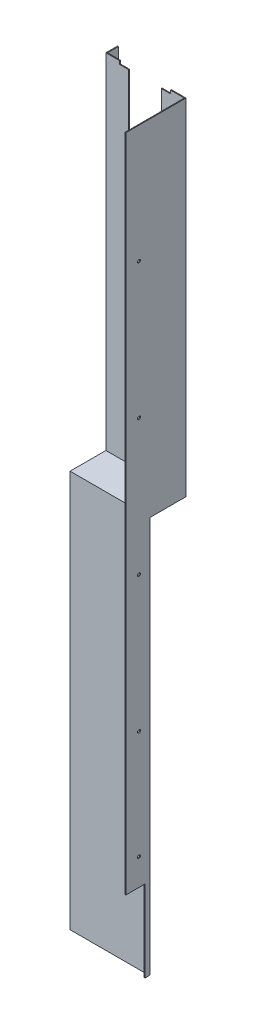
SolidWorks part; units mm, degrees
ref_plane "前视基准面" through (0, 0, 0) normal (0, 0, 1) x (1, 0, 0)
ref_plane "上视基准面" through (0, 0, 0) normal (0, 1, 0) x (1, 0, 0)
ref_plane "右视基准面" through (0, 0, 0) normal (1, 0, 0) x (0, 0, -1)
sketch "草图1" plane through (0, 0, 0) normal (0, 0, 1) x (1, 0, 0)
  line L1 (0, 0) -> (146, 0)
  line L2 (0, 0) -> (0, 636)
  line L3 (0, 636) -> (146, 636)
  line L4 (146, 0) -> (146, 636)
  dimension "D1" = 146
  dimension "D2" = 636
extrude "凸台-拉伸1" add sketch "草图1" along normal blind 1.5
sketch "草图3" plane through (0, 0, 1.5) normal (0, 0, 1) x (1, 0, 0)
  line L0 (0, 0) -> (146, 0) construction
  line L1 (146, 636) -> (144.5, 636)
  line L2 (146, 636) -> (146, 0)
  line L3 (146, 0) -> (144.5, 0)
  line L4 (144.5, 636) -> (144.5, 0)
  dimension "D1" = 1.5
extrude "凸台-拉伸3" add sketch "草图3" along normal blind 109
sketch "草图4" plane through (0, 0, 1.5) normal (0, 0, 1) x (1, 0, 0)
  line L0 (144.5, 636) -> (144.5, 0) construction
  line L1 (0, 0) -> (144.5, 0)
  line L2 (0, 0) -> (0, 1.5)
  line L3 (0, 1.5) -> (144.5, 1.5)
  line L4 (144.5, 0) -> (144.5, 1.5)
  dimension "D1" = 1.5
extrude "凸台-拉伸4" add sketch "草图4" along normal blind 66
sketch "草图5" plane through (0, 0, 0) normal (0, -1, 0) x (1, 0, 0)
  line L0 (0, 67.5) -> (144.5, 67.5)
  line L1 (0, 67.5) -> (144.5, 67.5) construction
  line L2 (144.5, 110.5) -> (144.5, 67.5) construction
  line L3 (144.5, 67.5) -> (144.5, 110.5)
  line L4 (144.5, 110.5) -> (146, 110.5)
  line L5 (146, 110.5) -> (146, 66)
  line L6 (146, 110.5) -> (146, 0) construction
  line L7 (146, 66) -> (0, 66)
  line L8 (0, 67.5) -> (0, 0) construction
  line L9 (0, 66) -> (0, 67.5)
  dimension "D1" = 1.5
extrude "凸台-拉伸5" add sketch "草图5" along normal blind 730
sketch "草图6" plane through (0, 0, 0) normal (0, 0, -1) x (-1, 0, 0)
  line L1 (0, 636) -> (-1.5, 636)
  line L2 (0, 636) -> (0, 1.5)
  line L3 (0, 1.5) -> (-1.5, 1.5)
  line L4 (-1.5, 636) -> (-1.5, 1.5)
  line L5 (0, 0) -> (-146, 0) construction
  dimension "D1" = 1.5
  dimension "D2" = 1.5
extrude "凸台-拉伸6" add sketch "草图6" along normal blind 20
sketch "草图7" plane through (0, 0, 66) normal (0, 0, -1) x (-1, 0, 0)
  line L0 (0, -730) -> (-146, -730) construction
  line L1 (0, 0) -> (-1.5, 0)
  line L2 (0, 0) -> (0, -730)
  line L3 (0, -730) -> (-1.5, -730)
  line L4 (-1.5, 0) -> (-1.5, -730)
  dimension "D1" = 1.5
extrude "凸台-拉伸7" add sketch "草图7" along normal blind 10
sketch "草图8" plane through (0, 0, 0) normal (0, -1, 0) x (1, 0, 0)
  line L1 (1.5, 56) -> (0, 56)
  line L2 (1.5, 56) -> (1.5, 0)
  line L3 (1.5, 0) -> (0, 0)
  line L4 (0, 56) -> (0, 0)
extrude "凸台-拉伸8" add sketch "草图8" along normal blind 10
sketch "草图9" plane through (144.5, 0, 0) normal (-1, 0, 0) x (0, 0, 1)
  line L1 (110.5, -730) -> (75.5, -730)
  line L2 (110.5, -730) -> (110.5, -580)
  line L3 (110.5, -580) -> (75.5, -580)
  line L4 (75.5, -730) -> (75.5, -580)
  dimension "D1" = 150
  dimension "D2" = 35
extrude "切除-拉伸1" cut sketch "草图9" against normal blind 2
sketch "草图10" plane through (0, 0, 1.5) normal (0, 0, 1) x (1, 0, 0)
  line L0 (0, 636) -> (0, 1.5) construction
  line L1 (25, 636) -> (119, 636)
  line L2 (119, 636) -> (119, 630)
  line L3 (25, 630) -> (42, 630)
  line L4 (25, 636) -> (25, 630)
  line L6 (42, 630) -> (42, 501)
  line L7 (42, 501) -> (102, 501)
  line L8 (102, 630) -> (102, 501)
  line L9 (102, 630) -> (119, 630)
  dimension "D1" = 94
  dimension "D2" = 6
  dimension "D3" = 60
  dimension "D4" = 17
  dimension "D5" = 135
  dimension "D6" = 17
  dimension "D7" = 25
extrude "切除-拉伸2" cut sketch "草图10" against normal blind 2
hole_wizard "Ø5.5 (5.5) 直径孔1" positions "草图12" profile "草图11" hole size "Ø5.5" standard "GB" end condition through all
sketch "草图12" plane through (144.5, 0, 0) normal (-1, 0, 0) x (0, 0, 1)
  line L1 (86.5, 636) -> (86.5, -907.068) construction
  line L2 (110.5, 636) -> (1.5, 636) construction
  line L4 (110.5, 636) -> (110.5, -580) construction
  point P0 (86.5, 419)
  point P1 (86.5, 169)
  point P3 (86.5, -81)
  point P5 (86.5, -331)
  point P13 (86.5, -531)
  dimension "D1" = 24
  dimension "D2" = 217
  dimension "D3" = 250
  dimension "D4" = 250
  dimension "D5" = 250
  dimension "D6" = 200
sketch "草图11" plane through (144.5, 419, 86.5) normal (0, 1, 0) x (0, 0, 1)
  line L0 (0, 0) -> (0, 1.5001)
  line L1 (0, 1.5001) -> (2.75, 1.5001)
  line L2 (2.75, 1.5001) -> (2.75, 0)
  line L5 (2.75, 0) -> (0, 0)
  line L11 (0, -6.35) -> (0, 107.95) construction
  dimension "通孔孔直径" = 5.5
  dimension "通孔孔深度" = 1.5001
hole_wizard "Ø5.5 (5.5) 直径孔2" positions "草图14" profile "草图13" hole size "Ø5.5" standard "GB" end condition through all
sketch "草图14" plane through (0, 0, 0) normal (-1, 0, 0) x (0, 0, 1)
  line L0 (-10, 636) -> (-10, -161.2553) construction
  line L1 (1.5, 636) -> (-20, 636) construction
  line L3 (-20, 1.5) -> (-20, 636) construction
  line L4 (-20, 1.5) -> (0, 1.5) construction
  point P0 (-10, 301.5)
  point P1 (-10, 101.5)
  dimension "D1" = 10
  dimension "D2" = 200
  dimension "D3" = 100
sketch "草图13" plane through (0, 301.5, -10) normal (0, 1, 0) x (0, 0, 1)
  line L0 (0, 0) -> (0, 146.0001)
  line L1 (0, 146.0001) -> (2.75, 146.0001)
  line L2 (2.75, 146.0001) -> (2.75, 0)
  line L5 (2.75, 0) -> (0, 0)
  line L11 (0, -6.35) -> (0, 107.95) construction
  dimension "通孔孔直径" = 5.5
  dimension "通孔孔深度" = 146.0001
